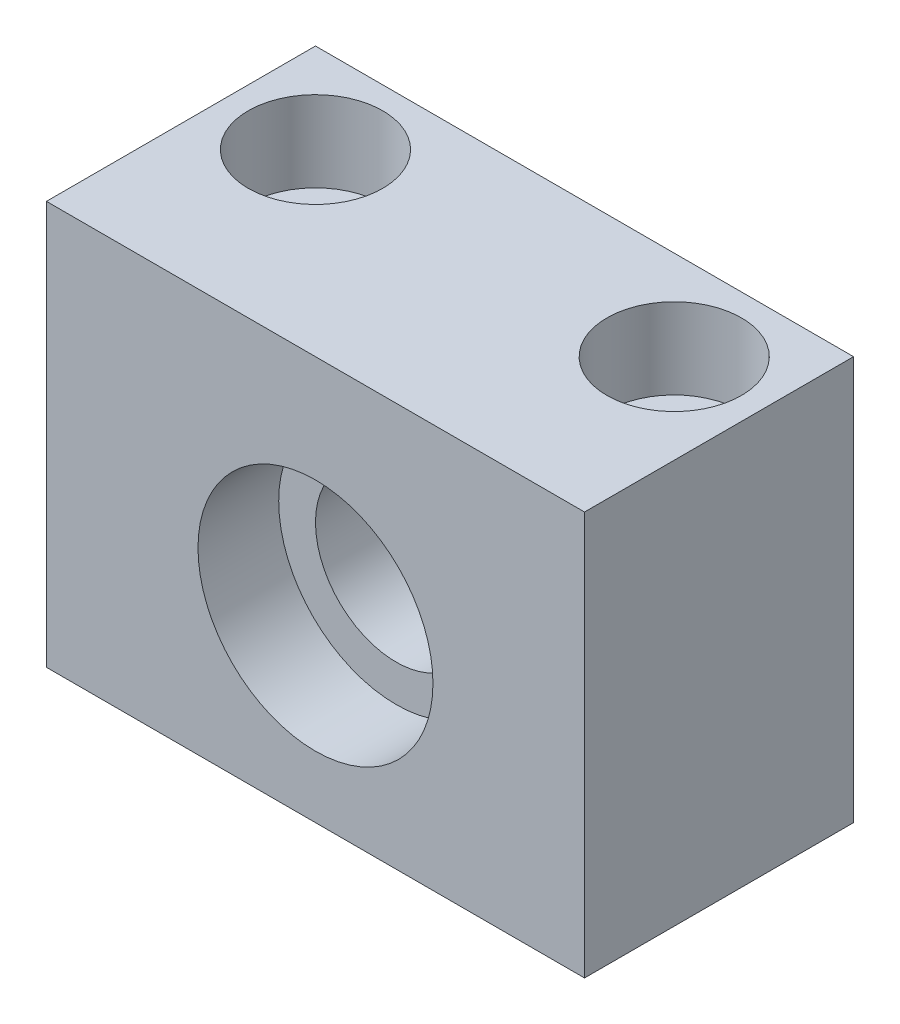
SolidWorks part; units mm, degrees
ref_plane "Front Plane" through (0, 0, 0) normal (0, 0, 1) x (1, 0, 0)
ref_plane "Top Plane" through (0, 0, 0) normal (0, 1, 0) x (1, 0, 0)
ref_plane "Right Plane" through (0, 0, 0) normal (1, 0, 0) x (0, 0, -1)
sketch "Sketch1" plane through (0, 0, 0) normal (0, 0, 1) x (1, 0, 0)
  line L1 (-30, -20) -> (30, -20)
  line L2 (-30, -20) -> (-30, 25)
  line L3 (-30, 25) -> (30, 25)
  line L4 (30, -20) -> (30, 25)
  circle A0 centre (0, 0) radius 9
  dimension "D1" = 18
  dimension "D2" = 20
  dimension "D3" = 45
  dimension "D4" = 30
  dimension "D5" = 60
extrude "Boss-Extrude1" add sketch "Sketch1" along normal blind 30
hole_wizard "Hole size per socket head cap screw type1" positions "草图3" profile "草图2" counterbore size "M8" standard "GB" end condition through all
sketch "草图3" plane through (0, 25, 0) normal (0, 1, 0) x (-1, 0, 0)
  line L2 (30, 30) -> (30, 0) construction
  line L3 (-30, 0) -> (30, 0) construction
  point P0 (20, 10)
  point P1 (-20, 10)
  dimension "D1" = 40
  dimension "D2" = 10
  dimension "D3" = 10
sketch "草图2" plane through (-20, 25, 10) normal (1, 0, 0) x (0, 0, 1)
  line L0 (0, 0) -> (0, 45)
  line L1 (0, 45) -> (4.5, 45)
  line L3 (4.5, 45) -> (4.5, 9)
  line L4 (4.5, 9) -> (7.5, 9)
  line L5 (7.5, 9) -> (7.5, 0)
  line L7 (7.5, 0) -> (0, 0)
  line L11 (0, -6.35) -> (0, 107.95) construction
  dimension "通孔孔直径" = 9
  dimension "通孔孔深度" = 45
  dimension "柱形沉头孔直径" = 15
  dimension "柱形沉头孔深度" = 9
sketch "Sketch2" plane through (0, 0, 30) normal (0, 0, 1) x (1, 0, 0)
  circle A0 centre (0, 0) radius 13.1
  dimension "D1" = 26.2
extrude "Extrude1" cut sketch "Sketch2" against normal blind 9
sketch "Sketch3" plane through (0, 0, 0) normal (0, 0, -1) x (-1, 0, 0)
  circle A0 centre (0, 0) radius 13.1
  dimension "D1" = 26.2
extrude "Extrude2" cut sketch "Sketch3" against normal blind 9
